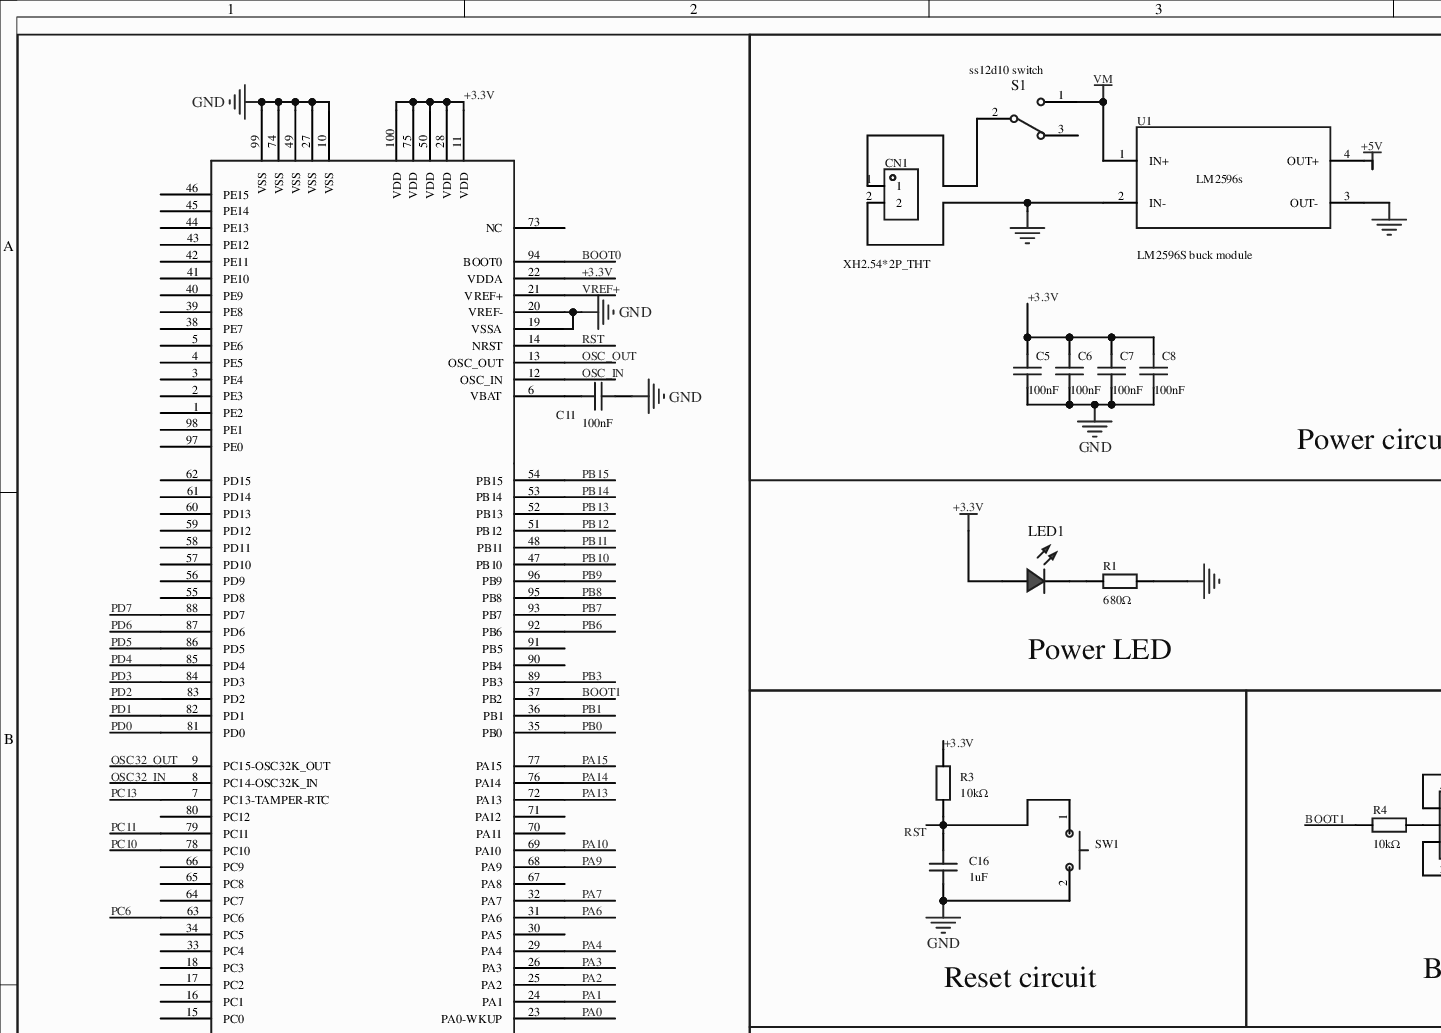
[diagram p0: MISC62445-3.schdoc, top left]
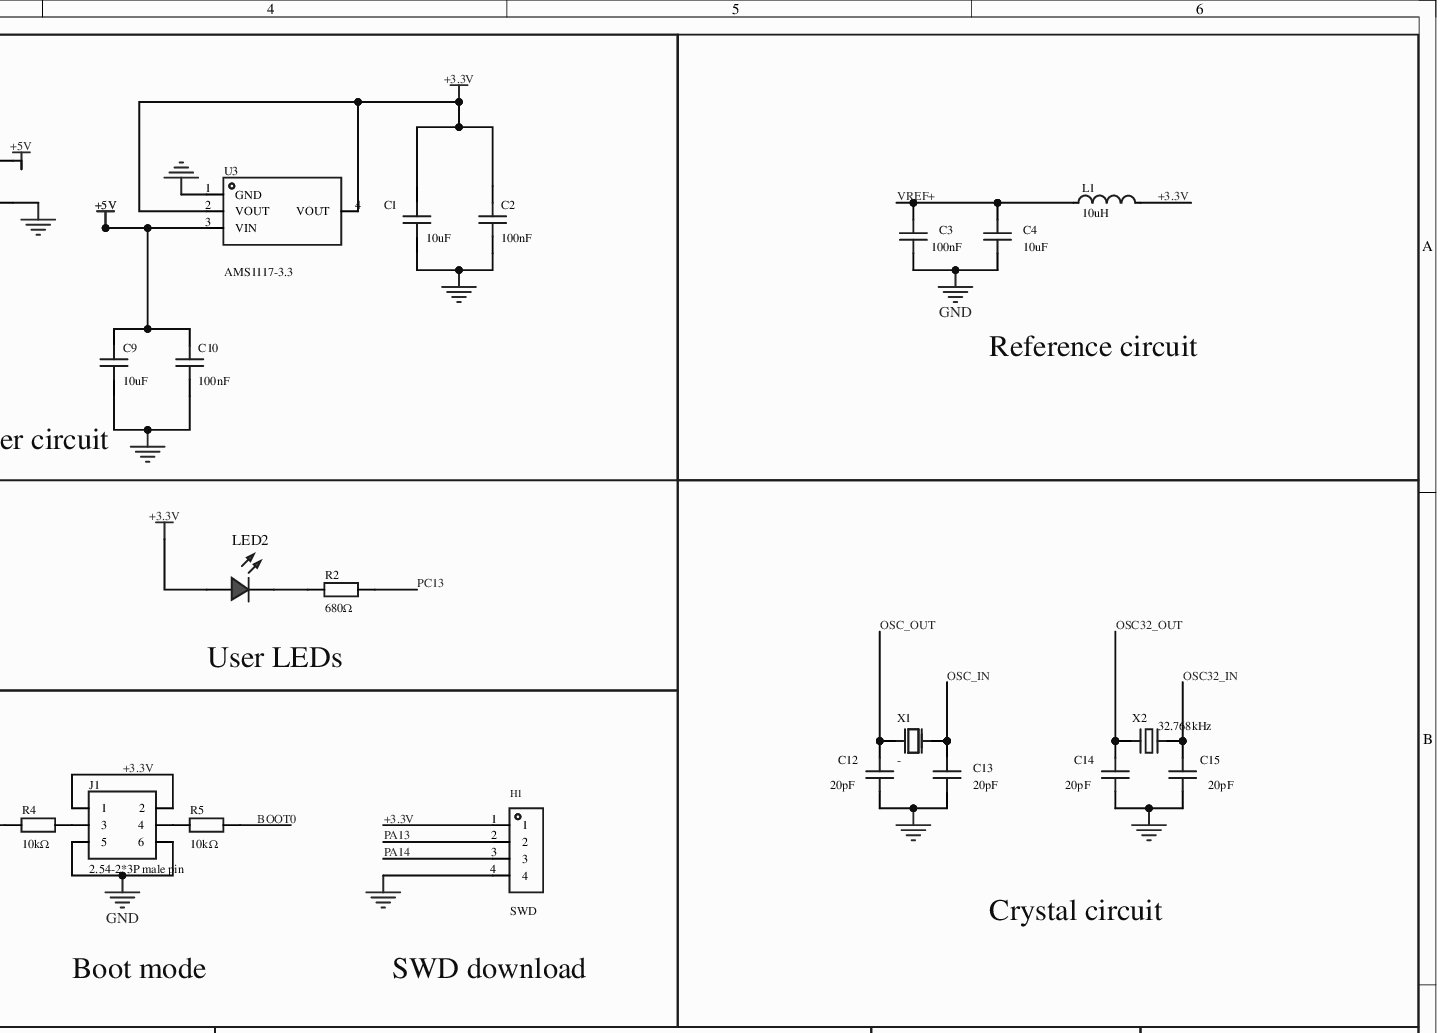
[diagram p1: MISC62445-3.schdoc, top right]
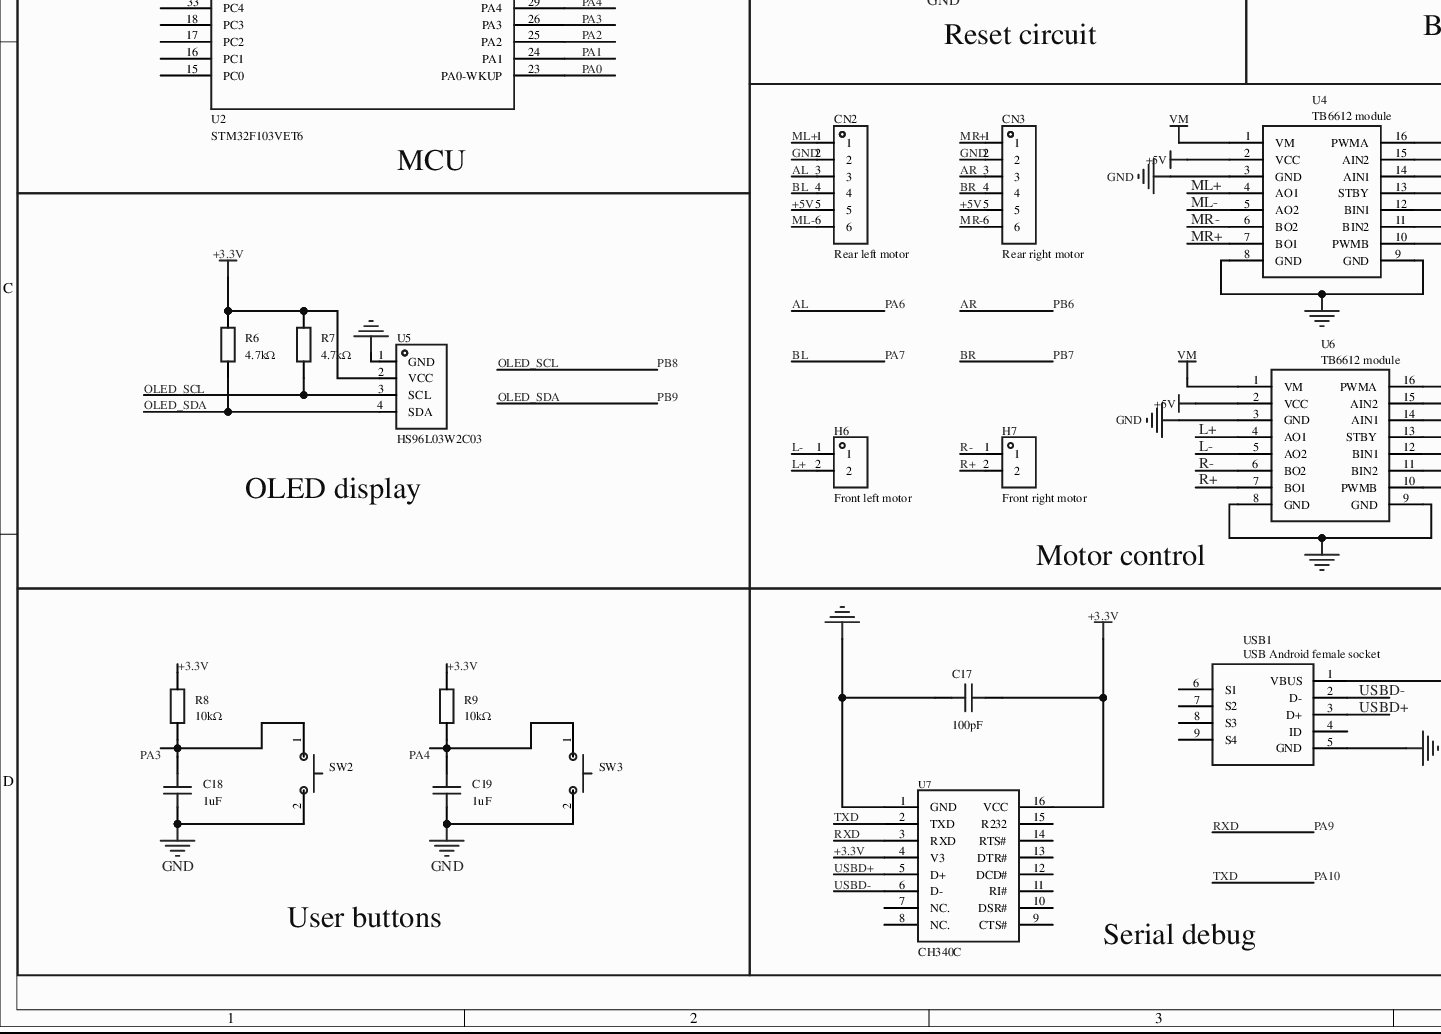
[diagram p2: MISC62445-3.schdoc, bottom left]
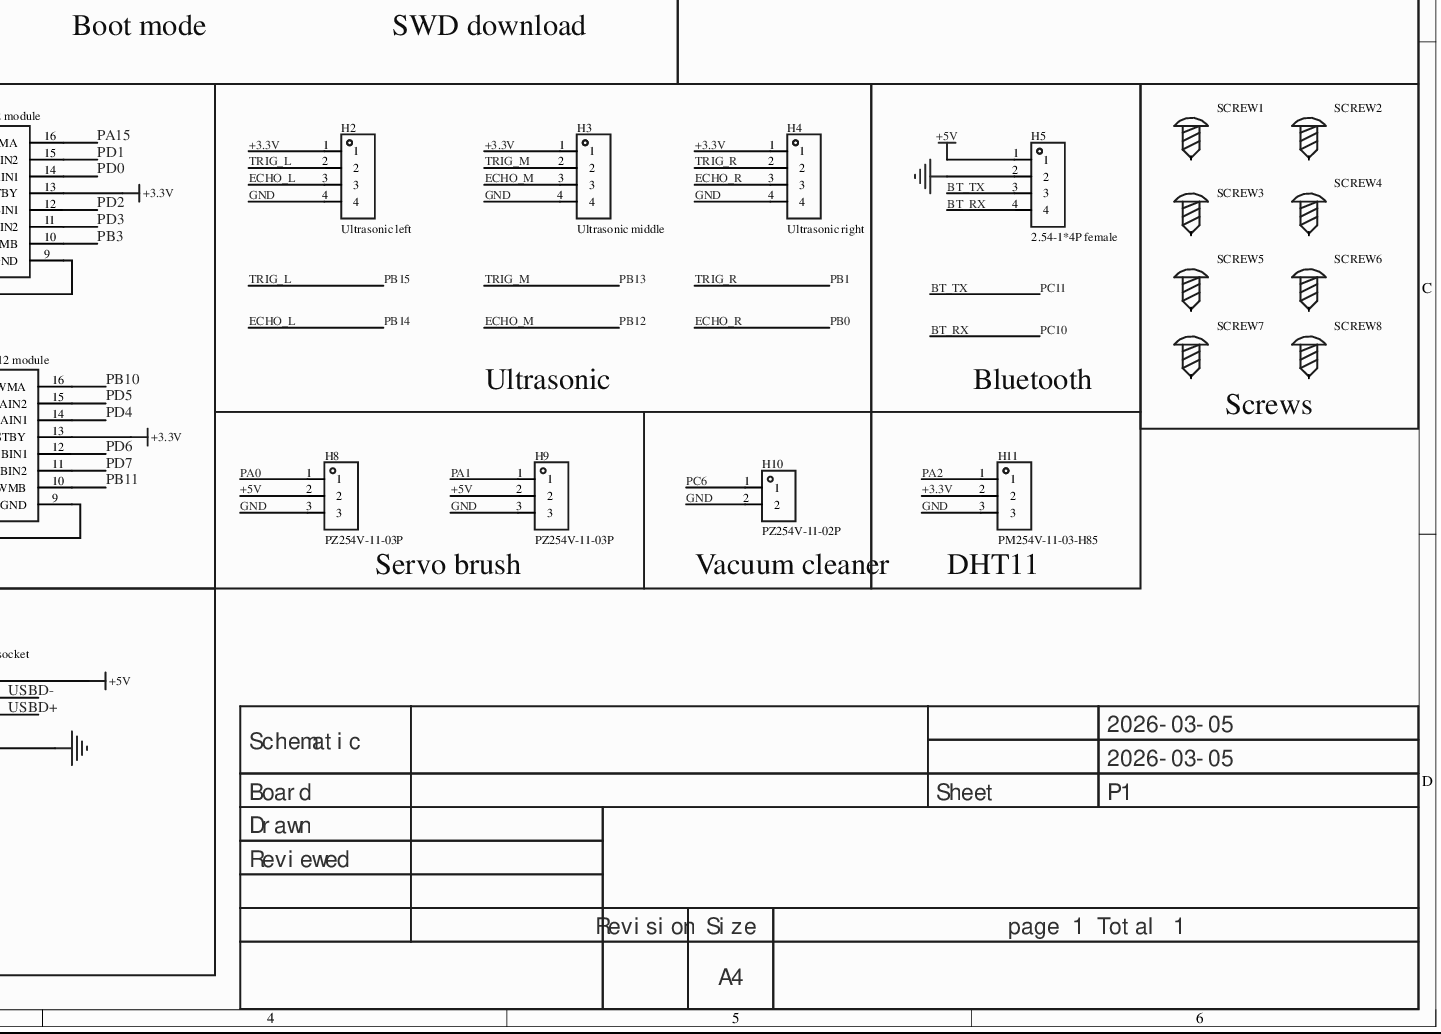
[diagram p3: MISC62445-3.schdoc, bottom right]
# Altium project MISC62445-2.PrjPcb
1 sheet, 68 parts. Net scope: global (net labels, ports and power ports of the same name join across sheets).
Board file: MISC62445.pcbdoc

## Sheet MISC62445-3.schdoc
size 420 x 297 mm; Version: V1.0; @Project Name: MISC62445; @Page Count: 1; @Update Date: 2026-03-05; @Create Date: 2026-03-05; @Schematic Name: MISC62445; @Page No: 1; @Create Time: 17:18:42; @Update Time: 10:03:47; @Board Name: MISC62445

### Parts
C1  10uF  [C0805]
C2  100nF  [C0805]
C3  100nF  [C0603]
C4  10uF  [C0603]
C5  100nF  [C0603]
C6  100nF  [C0603]
C7  100nF  [C0603]
C8  100nF  [C0603]
C9  10uF  [C0805]
C10  100nF  [C0805]
C11  100nF  [C0603]
C12  20pF  [C0805]
C13  20pF  [C0805]
C14  20pF  [C0805]
C15  20pF  [C0805]
C16  1uF  [C0603]
C17  100pF  [C0805]
C18  1uF  [C0603]
C19  1uF  [C0603]
CN1  XH2.54*2P_THT  [CONN-TH_2P-P2.50-XH2.54-2P]
CN2  Rear left motor  [CONN-TH_XH2.54-6P]
CN3  Rear right motor  [CONN-TH_XH2.54-6P]
H1  SWD  [HDR-TH_4P-P2.54-V-M]
H2  Ultrasonic left  [HDR-TH_4P-P2.54-V-M]
H3  Ultrasonic middle  [HDR-TH_4P-P2.54-V-M]
H4  Ultrasonic right  [HDR-TH_4P-P2.54-V-M]
H5  2.54-1*4P female  [HDR-TH_4P-P2.54-V-F]
H6  Front left motor  [HDR-TH_2P-P2.54-V-M]
H7  Front right motor  [HDR-TH_2P-P2.54-V-M]
H8  PZ254V-11-03P  [HDR-TH_3P-P2.54-V-M]
H9  PZ254V-11-03P  [HDR-TH_3P-P2.54-V-M]
H10  PZ254V-11-02P  [HDR-TH_2P-P2.54-V-M]
H11  PM254V-11-03-H85  [HDR-TH_3P-P2.54-V-F]
J1  2.54-2*3P male pin  [HDR-TH_6P-P2.54-V-M-R2-C3-S2.54-1]
L1  10uH  [L0603]
LED1  NCD0805R1  [LED0805-RD_RED]  (value not drawn)
LED2  NCD0805R1  [LED0805-RD_RED]  (value not drawn)
R1  680Ω  [R0805]
R2  680Ω  [R0805]
R3  10kΩ  [R0603]
R4  10kΩ  [R0603]
R5  10kΩ  [R0603]
R6  4.7kΩ  [R0805]
R7  4.7kΩ  [R0805]
R8  10kΩ  [R0603]
R9  10kΩ  [R0603]
S1  ss12d10 switch  [SS12D10]
SCREW1  (no value)  [M3螺丝]
SCREW2  (no value)  [M3螺丝]
SCREW3  (no value)  [M3螺丝]
SCREW4  (no value)  [M3螺丝]
SCREW5  (no value)  [M2螺丝]
SCREW6  (no value)  [M2螺丝]
SCREW7  (no value)  [M2螺丝]
SCREW8  (no value)  [M2螺丝]
SW1  1TS002C-2300-4300-CT  [SW-SMD_L6.0-W3.5-LS8.0-EH]  (value not drawn)
SW2  1TS002C-2300-4300-CT  [SW-SMD_L6.0-W3.5-LS8.0-EH]  (value not drawn)
SW3  1TS002C-2300-4300-CT  [SW-SMD_L6.0-W3.5-LS8.0-EH]  (value not drawn)
U1  LM2596S buck module  [LM2596S]
U2  STM32F103VET6  [LQFP-100_L14.0-W14.0-P0.50-LS16.0-BL]
U3  AMS1117-3.3  [SOT-223-3_L6.5-W3.4-P2.30-LS7.0-BR]
U4  TB6612 module  [TB6612-2X8]
U5  HS96L03W2C03  [OLED-TH_L27.8-W27.2-P2.54_C9900033791]
U6  TB6612 module  [TB6612-2X8]
U7  CH340C  [SOP-16_L10.0-W3.9-P1.27-LS6.0-BL]
USB1  USB Android female socket  [MICRO-USB-SMD_MICRO-USB-A8]
X1  -  [HC-49US_L11.5-W4.5-P4.88]
X2  32.768kHz  [OSC-SMD_L3.2-W1.5]

### Blocks framed on the sheet
MCU: C11 U2
Power circuit: C1 C2 C5-C10 CN1 S1 U1 U3
Reference circuit: C3 C4 L1
Crystal circuit: C12-C15 X1 X2
Reset circuit: C16 R3 SW1
Motor control: CN2 CN3 H6 H7 U4 U6
Ultrasonic: H2-H4
Bluetooth: H5
Screws: SCREW1-SCREW8
Vacuum cleaner: H10
User buttons: C18 C19 R8 R9 SW2 SW3

### Nets
+3.3V: C1.2 C2.2 C5.1 C6.1 C7.1 C8.1 C17.2 H1.1 H2.1 H3.1 H4.1 H11.2 J1.1 J1.2 L1.2 LED1.2(A) LED2.2(A) R3.2 R6.1 R7.1 R8.2 R9.2 U2.11(VDD) U2.22(VDDA) U2.28(VDD) U2.50(VDD) U2.75(VDD) U2.100(VDD) U3.2(VOUT) U3.4(VOUT) U4.13(STBY) U5.2(VCC) U6.13(STBY) U7.4(V3) U7.16(VCC)
+5V: C9.2 C10.2 CN2.5 CN3.5 H5.1 H8.2 H9.2 U1.4(OUT+) U3.3(VIN) U4.2(VCC) U6.2(VCC) USB1.1(VBUS)
GND: C1.1 C2.1 C3.1 C4.1 C5.2 C6.2 C7.2 C8.2 C9.1 C10.1 C11.2 C12.1 C13.1 C14.1 C15.1 C16.1 C17.1 C18.1 C19.1 CN1.2 CN2.2 CN3.2 H1.4 H2.4 H3.4 H4.4 H5.2 H8.3 H9.3 H10.2 H11.3 J1.5 J1.6 R1.2 SW1.2(B) SW2.2(B) SW3.2(B) U1.2(IN-) U1.3(OUT-) U2.10(VSS) U2.19(VSSA) U2.20(VREF-) U2.27(VSS) U2.49(VSS) U2.74(VSS) U2.99(VSS) U3.1(GND) U4.3(GND) U4.8(GND) U4.9(GND) U5.1(GND) U6.3(GND) U6.8(GND) U6.9(GND) U7.1(GND) USB1.5(GND)
VM: S1.1 U1.1(IN+) U4.1(VM) U6.1(VM)
AL: CN2.3 U2.31(PA6)  [also labelled PA6]
AR: CN3.3 U2.92(PB6)  [also labelled PB6]
BL: CN2.4 U2.32(PA7)  [also labelled PA7]
BOOT0: R5.2 U2.94(BOOT0)
BOOT1: R4.1 U2.37(PB2)
BR: CN3.4 U2.93(PB7)  [also labelled PB7]
BT_RX: H5.4 U2.78(PC10)  [also labelled PC10]
BT_TX: H5.3 U2.79(PC11)  [also labelled PC11]
ECHO_L: H2.3 U2.53(PB14)  [also labelled PB14]
ECHO_M: H3.3 U2.51(PB12)  [also labelled PB12]
ECHO_R: H4.3 U2.35(PB0)  [also labelled PB0]
L+: H6.2 U6.4(AO1)
L-: H6.1 U6.5(AO2)
ML+: CN2.1 U4.4(AO1)
ML-: CN2.6 U4.5(AO2)
MR+: CN3.1 U4.7(BO1)
MR-: CN3.6 U4.6(BO2)
OLED_SCL: R7.2 U2.95(PB8) U5.3(SCL)  [also labelled PB8]
OLED_SDA: R6.2 U2.96(PB9) U5.4(SDA)  [also labelled PB9]
OSC32_IN: C15.2 U2.8(PC14-OSC32K_IN) X2.2
OSC32_OUT: C14.2 U2.9(PC15-OSC32K_OUT) X2.1
OSC_IN: C13.2 U2.12(OSC_IN) X1.2(OSC2)
OSC_OUT: C12.2 U2.13(OSC_OUT) X1.1(OSC1)
PA0: H8.1 U2.23(PA0-WKUP)
PA1: H9.1 U2.24(PA1)
PA2: H11.1 U2.25(PA2)
PA3: C18.2 R8.1 SW2.1(A) U2.26(PA3)
PA4: C19.2 R9.1 SW3.1(A) U2.29(PA4)
PA9: U2.68(PA9) U7.3(RXD)  [also labelled RXD]
PA10: U2.69(PA10) U7.2(TXD)  [also labelled TXD]
PA13: H1.2 U2.72(PA13)
PA14: H1.3 U2.76(PA14)
PA15: U2.77(PA15) U4.16(PWMA)
PB1: H4.2 U2.36(PB1)  [also labelled TRIG_R]
PB3: U2.89(PB3) U4.10(PWMB)
PB10: U2.47(PB10) U6.16(PWMA)
PB11: U2.48(PB11) U6.10(PWMB)
PB13: H3.2 U2.52(PB13)  [also labelled TRIG_M]
PB15: H2.2 U2.54(PB15)  [also labelled TRIG_L]
PC6: H10.1 U2.63(PC6)
PC13: R2.2 U2.7(PC13-TAMPER-RTC)
PD0: U2.81(PD0) U4.14(AIN1)
PD1: U2.82(PD1) U4.15(AIN2)
PD2: U2.83(PD2) U4.12(BIN1)
PD3: U2.84(PD3) U4.11(BIN2)
PD4: U2.85(PD4) U6.14(AIN1)
PD5: U2.86(PD5) U6.15(AIN2)
PD6: U2.87(PD6) U6.12(BIN1)
PD7: U2.88(PD7) U6.11(BIN2)
R+: H7.2 U6.7(BO1)
R-: H7.1 U6.6(BO2)
RST: C16.2 R3.1 SW1.1(A) U2.14(NRST)
USBD+: U7.5(D+) USB1.3(D+)
USBD-: U7.6(D-) USB1.2(D-)
VREF+: C3.2 C4.2 L1.1 U2.21(VREF+)
NetC11_1: C11.1 U2.6(VBAT)
NetCN1_1: CN1.1 S1.2
NetJ1_3: J1.3 R4.2
NetJ1_4: J1.4 R5.1
NetLED1_1: LED1.1(C) R1.1
NetLED2_1: LED2.1(C) R2.1

Not connected (* = marked no-connect by the designer): S1 3*; SCREW1 1*; SCREW2 1*; SCREW3 1*; SCREW4 1*; SCREW5 1*; SCREW6 1*; SCREW7 1*; SCREW8 1*; U2 1(PE2)* 2(PE3)* 3(PE4)* 4(PE5)* 5(PE6)* 15(PC0)* 16(PC1)* 17(PC2)* 18(PC3)* 30(PA5)* 33(PC4)* 34(PC5)* 38(PE7)* 39(PE8)* 40(PE9)* 41(PE10)* 42(PE11)* 43(PE12)* 44(PE13)* 45(PE14)* 46(PE15)* 55(PD8)* 56(PD9)* 57(PD10)* 58(PD11)* 59(PD12)* 60(PD13)* 61(PD14)* 62(PD15)* 64(PC7)* 65(PC8)* 66(PC9)* 67(PA8)* 70(PA11)* 71(PA12)* 73(NC)* 80(PC12)* 90(PB4)* 91(PB5)* 97(PE0)* 98(PE1)*; U7 7(NC.)* 8(NC.)* 9(CTS#)* 10(DSR#)* 11(RI#)* 12(DCD#)* 13(DTR#)* 14(RTS#)* 15(R232)*; USB1 4(ID)* 6(S1)* 7(S2)* 8(S3)* 9(S4)*

### Notes on the sheet
- Power LED
- User LEDs
- Boot mode
- SWD download
- (near U5) OLED display
- (near H9) Servo brush
- (near H11) DHT11
- Serial debug
- 2026-03-05
- Schematic
- Board
- Sheet
- P1
- Drawn
- Reviewed
- Revision
- Size
- A4
- page 1 Total 1

### Library data of the parts
C1 C9 = GRM21BR61H106KE43L: Capacitance:10uF;Tolerance:±10%;Rated voltage:50V;Dielectric (temp. coeff.):X5R;; Manufacturer: muRata(村田); AddInBom: yes; ModelId: 1ba041120af144c991958decab20d241; ModelName: C0805_L2.0-W1.3-H1.3; ModelTransform: 78.74,51.181,0,0,0,0,0,0.0005,0; Tolerance: ±10%; Voltage Rated: 50V; Temperature Coefficient: X5R; Symbol: CapAcitance; Device: GRM21BR61H106KE43L; LCSC Part Name: 10uF ±10% 50V; SupplierPart: C440198; ManufacturerPart: GRM21BR61H106KE43L; Supplier Footprint: 0805; JLCPCB Part Class: Basic Part; Datasheet: https://example.com/upload/public/pdf/source/20230811/95AAE0C9AF55EDC31B7A4D8B733F534E.pdf; Supplier: LCSC; ConvertToPcb: yes; FootprintName: C0805; Value: 10uF
C2 C10 = CL21B104KBCNNNC: Capacitance:100nF;Tolerance:±10%;Rated voltage:50V;Dielectric (temp. coeff.):X7R;; Manufacturer: SAMSUNG(三星); AddInBom: yes; ModelId: 1ba041120af144c991958decab20d241; ModelName: C0805_L2.0-W1.3-H1.3; ModelTransform: 78.74,51.181,0,0,0,0,0,0.0005,0; Tolerance: ±10%; Voltage Rated: 50V; Temperature Coefficient: X7R; Symbol: CapAcitance; Device: CL21B104KBCNNNC; LCSC Part Name: 100nF ±10% 50V; SupplierPart: C1711; ManufacturerPart: CL21B104KBCNNNC; Supplier Footprint: 0805; JLCPCB Part Class: Extended Part; Datasheet: https://example.com/upload/public/pdf/source/20160218/1457707763339.pdf; Supplier: LCSC; ConvertToPcb: yes; FootprintName: C0805; Value: 100nF
C3 C5-C8 C11 = CC0603KRX7R9BB104: Capacitance:100nF;Tolerance:±10%;Rated voltage:50V;Dielectric (temp. coeff.):X7R;; Manufacturer: YAGEO(国巨); Check: true; AddInBom: yes; ModelId: ac125912035d415993ca9572d50418b1; ModelName: C0603_L1.6-W0.8-H0.8; ModelTransform: 62.992,31.496,0,0,0,0,0,0,0; Tolerance: ±10%; Voltage Rated: 50V; Temperature Coefficient: X7R; Symbol: CapAcitance; Device: CC0603KRX7R9BB104; Supplier Part: C14663; LCSC Part Name: 100nF ±10% 50V; ManufacturerPart: CC0603KRX7R9BB104; Supplier Footprint: 0603; JLCPCB Part Class: Basic Part; Datasheet: https://example.com/upload/public/pdf/source/20180910/C282072_33301C7F631E79921B82A8DAC6BCC5B3.pdf; Supplier: LCSC; ConvertToPcb: yes; FootprintName: C0603; Value: 100nF
C4 = CL10A106KP8NNNC: Capacitance:10uF;Tolerance:±10%;Rated voltage:10V;Dielectric:X5R;; Manufacturer: SAMSUNG(三星); Check: true; AddInBom: yes; ModelId: ac125912035d415993ca9572d50418b1; ModelName: C0603_L1.6-W0.8-H0.8; ModelTransform: 62.992,31.496,0,0,0,0,0,0,0; Tolerance: ±10%; Voltage Rated: 10V; Temperature Coefficient: X5R; Symbol: CapAcitance; Device: CL10A106KP8NNNC; Supplier Part: C19702; LCSC Part Name: 10uF ±10% 10V; ManufacturerPart: CL10A106KP8NNNC; Supplier Footprint: 0603; JLCPCB Part Class: Basic Part; Datasheet: https://example.com/upload/public/pdf/source/20160103/1457707703378.pdf; Supplier: LCSC; ConvertToPcb: yes; FootprintName: C0603; Value: 10uF
C12-C15 = CL21C200JBANNNC: Capacitance:20pF;Tolerance:±5%;Rated voltage:50V;Dielectric:C0G;; Manufacturer: SAMSUNG(三星); AddInBom: yes; ModelId: 1ba041120af144c991958decab20d241; ModelName: C0805_L2.0-W1.3-H1.3; ModelTransform: 78.74,51.181,0,0,0,0,0,0.0005,0; Tolerance: ±5%; Voltage Rated: 50V; Temperature Coefficient: C0G; Symbol: CapAcitance; Device: CL21C200JBANNNC; LCSC Part Name: 20pF ±5% 50V; SupplierPart: C1798; ManufacturerPart: CL21C200JBANNNC; Supplier Footprint: 0805; JLCPCB Part Class: Basic Part; Datasheet: https://example.com/upload/public/pdf/source/20160218/1457707763339.pdf; Supplier: LCSC; ConvertToPcb: yes; FootprintName: C0805; Value: 20pF
C16 C18 C19 = CL10A105KB8NNNC: Capacitance:1uF;Tolerance:±10%;Rated voltage:50V;Dielectric:X5R;; Manufacturer: SAMSUNG(三星); Check: true; AddInBom: yes; ModelId: ac125912035d415993ca9572d50418b1; ModelName: C0603_L1.6-W0.8-H0.8; ModelTransform: 62.992,31.496,0,0,0,0,0,0,0; Tolerance: ±10%; Voltage Rated: 50V; Temperature Coefficient: X5R; Symbol: CapAcitance; Device: CL10A105KB8NNNC; Supplier Part: C15849; LCSC Part Name: 1uF ±10% 50V; ManufacturerPart: CL10A105KB8NNNC; Supplier Footprint: 0603; JLCPCB Part Class: Basic Part; Datasheet: https://example.com/upload/public/pdf/source/20160103/1457707679084.pdf; Supplier: LCSC; ConvertToPcb: yes; FootprintName: C0603; Value: 1uF
C17 = CL21C101JBANNNC: Capacitance:100pF;Tolerance:±5%;Rated voltage:50V;Dielectric:C0G;; Manufacturer: SAMSUNG(三星); AddInBom: yes; ModelId: 1ba041120af144c991958decab20d241; ModelName: C0805_L2.0-W1.3-H1.3; ModelTransform: 78.74,51.181,0,0,0,0,0,0.0005,0; Tolerance: ±5%; Voltage Rated: 50V; Temperature Coefficient: C0G; Symbol: CapAcitance; Device: CL21C101JBANNNC; LCSC Part Name: 100pF ±5% 50V; SupplierPart: C1790; ManufacturerPart: CL21C101JBANNNC; Supplier Footprint: 0805; JLCPCB Part Class: Basic Part; Datasheet: https://example.com/upload/public/pdf/source/20160218/1457707763339.pdf; Supplier: LCSC; ConvertToPcb: yes; FootprintName: C0805; Value: 100pF
CN1 = XH2.54*2P_直插: Manufacturer: null; Convert to PCB: yes; ModelId: 325c595e30db4df8abe76612dd40b0fa; Origin Footprint: CONN-TH_2P-P2.50-XH2.54-2P; Device: XH2.54*2P_THT; Symbol: XH2.54*2P_THT; Supplier: LCSC; Supplier Part: C9900008615; Manufacturer Part: XH2.54*2P_直插; JLCPCB Part Class: Extended Part; Add into BOM: yes; FootprintName: CONN-TH_2P-P2.50-XH2.54-2P; link: https://example.com/pdf/applyPasteComponent/2021-09-13/837084A/aaafcbedaa1341f78bdd46f8ab13ab21/XH2_54datasheet.pdf; 3DModel: CONN-TH_2P-P2.50-XH2.54-2P; ModelName: CONN-TH_2P-P2.50-XH2.54-2P
CN2 = XH2.54*6P_直插: Manufacturer Part: 后左电机; Symbol: XH2.54*6P_THT; AddInBom: yes; ModelId: a7224aacb0dc4305a7392217f7fd8fe2; ModelTransform: 688.975,224.409,0,0,0,0,-0.001,-17.719,-118.11; Device: XH2.54*6P_THT; LCSC Part Name: XH2.54*6P_直插; SupplierPart: C9900008614; Supplier Footprint: XH2.54_6P; JLCPCB Part Class: Extended library; Supplier: LCSC; ConvertToPcb: yes; FootprintName: CONN-TH_XH2.54-6P; ModelName: CONN-TH_XH2.54-6P
CN3 = XH2.54*6P_直插: Manufacturer Part: 后右电机; Symbol: XH2.54*6P_THT; AddInBom: yes; ModelId: a7224aacb0dc4305a7392217f7fd8fe2; ModelTransform: 688.975,224.409,0,0,0,0,-0.001,-17.719,-118.11; Device: XH2.54*6P_THT; LCSC Part Name: XH2.54*6P_直插; SupplierPart: C9900008614; Supplier Footprint: XH2.54_6P; JLCPCB Part Class: Extended library; Supplier: LCSC; ConvertToPcb: yes; FootprintName: CONN-TH_XH2.54-6P; ModelName: CONN-TH_XH2.54-6P
H1 = KH-2.54PH180-1X4P-L11.5: 排数:单排;总PIN位数:4P;间距:2.54mm;插针结构:1x4P;行距:-;安装类型:直插;圆针/方针:方针;额定电流:3A;额定电压:-;配合针长度:6mm;塑高:2.5mm;端接针长度:3mm;触头材质:-;工作温度范围:-40℃~+105℃;颜色:黑色;; Manufacturer: kinghelm(金航标); AddInBom: yes; ModelId: 112f4d05e8d64e99ab9a333894bea4f9; ModelName: HDR-TH_4P-P2.54-M-LI-1X4P; ModelTransform: 399.999,104.7242,0,0,0,0,0,0,-118.11; Pitch: 2.54mm; Pin Structure: 1x4P; Circluar Pins/Square Pins: Square pin; Current Rating (Max): 3A; Symbol: KH-2.54PH180-1X4P-L11.5; Manufacturer Part: SWD; Device: KH-2.54PH180-1X4P-L11.5; Supplier: LCSC; Supplier Part: C2905435; JLCPCB Part Class: Extended Part; LCSC Part Name: 2.54mm 1x4P 直插 方针; Supplier Footprint: 插件,P=2.54mm; Datasheet: https://example.com/upload/public/pdf/source/20211019/06FD9EA041E66F176E900F61FE678D35.pdf; ConvertToPcb: yes; FootprintName: HDR-TH_4P-P2.54-V-M; Number of Rows: Single row; Number of Pins: 4P; Row Spacing: -; Mounting Type: Through-hole; Voltage Rating (Max): -; Length of Mating Pin: 6mm; Insulation Height: 2.5mm; Length of End Connection Pin: 3mm; Contact Material: -; Operating Temperature Range: -40℃~+105℃; Color: Black
H2 = PZ254V-11-04P: 插针结构:1x4P;间距:2.54mm;行距:-;圆针/方针:方针;安装类型:直插;排数:单排;总PIN位数:4P;额定电流:3A;额定电压:250V;配合针长度:6mm;塑高:2.5mm;端接针长度:3mm;触头材质:-;工作温度范围:-40℃~+105℃;颜色:黑色;; Manufacturer Part: 超声波左; Manufacturer: XFCN(兴飞); Symbol: PZ254V-11-04P_C2691448; AddInBom: yes; ModelId: 112f4d05e8d64e99ab9a333894bea4f9; ModelName: HDR-TH_4P-P2.54-M-LI-1X4P; ModelTransform: 399.999,104.7242,0,0,0,0,0,0,-118.11; Pin Structure: 1x4P; Pitch: 2.54mm; Circluar Pins/Square Pins: Square pin; Current Rating (Max): 3A; Voltage Rating (Max): 250V; Device: PZ254V-11-04P; LCSC Part Name: 间距:2.54mm 1x4P 直插 方针; SupplierPart: C2691448; Supplier Footprint: 插件,P=2.54mm; JLCPCB Part Class: Extended library; Datasheet: https://example.com/upload/public/pdf/source/20200309/C492403_F9F19131791D08044AD4F84F8E751A34.pdf; Supplier: LCSC; ConvertToPcb: yes; FootprintName: HDR-TH_4P-P2.54-V-M; Row Spacing: -; Mounting Type: Through-hole; Number of Rows: Single row; Number of Pins: 4P; Length of Mating Pin: 6mm; Insulation Height: 2.5mm; Length of End Connection Pin: 3mm; Contact Material: -; Operating Temperature Range: -40℃~+105℃; Color: Black
H3 = PZ254V-11-04P: 插针结构:1x4P;间距:2.54mm;行距:-;圆针/方针:方针;安装类型:直插;排数:单排;总PIN位数:4P;额定电流:3A;额定电压:250V;配合针长度:6mm;塑高:2.5mm;端接针长度:3mm;触头材质:-;工作温度范围:-40℃~+105℃;颜色:黑色;; Manufacturer Part: 超声波中; Manufacturer: XFCN(兴飞); Symbol: PZ254V-11-04P_C2691448; AddInBom: yes; ModelId: 112f4d05e8d64e99ab9a333894bea4f9; ModelName: HDR-TH_4P-P2.54-M-LI-1X4P; ModelTransform: 399.999,104.7242,0,0,0,0,0,0,-118.11; Pin Structure: 1x4P; Pitch: 2.54mm; Circluar Pins/Square Pins: Square pin; Current Rating (Max): 3A; Voltage Rating (Max): 250V; Device: PZ254V-11-04P; LCSC Part Name: 间距:2.54mm 1x4P 直插 方针; SupplierPart: C2691448; Supplier Footprint: 插件,P=2.54mm; JLCPCB Part Class: Extended library; Datasheet: https://example.com/upload/public/pdf/source/20200309/C492403_F9F19131791D08044AD4F84F8E751A34.pdf; Supplier: LCSC; ConvertToPcb: yes; FootprintName: HDR-TH_4P-P2.54-V-M; Row Spacing: -; Mounting Type: Through-hole; Number of Rows: Single row; Number of Pins: 4P; Length of Mating Pin: 6mm; Insulation Height: 2.5mm; Length of End Connection Pin: 3mm; Contact Material: -; Operating Temperature Range: -40℃~+105℃; Color: Black
H4 = PZ254V-11-04P: 插针结构:1x4P;间距:2.54mm;行距:-;圆针/方针:方针;安装类型:直插;排数:单排;总PIN位数:4P;额定电流:3A;额定电压:250V;配合针长度:6mm;塑高:2.5mm;端接针长度:3mm;触头材质:-;工作温度范围:-40℃~+105℃;颜色:黑色;; Manufacturer Part: 超声波右; Manufacturer: XFCN(兴飞); Symbol: PZ254V-11-04P_C2691448; AddInBom: yes; ModelId: 112f4d05e8d64e99ab9a333894bea4f9; ModelName: HDR-TH_4P-P2.54-M-LI-1X4P; ModelTransform: 399.999,104.7242,0,0,0,0,0,0,-118.11; Pin Structure: 1x4P; Pitch: 2.54mm; Circluar Pins/Square Pins: Square pin; Current Rating (Max): 3A; Voltage Rating (Max): 250V; Device: PZ254V-11-04P; LCSC Part Name: 间距:2.54mm 1x4P 直插 方针; SupplierPart: C2691448; Supplier Footprint: 插件,P=2.54mm; JLCPCB Part Class: Extended library; Datasheet: https://example.com/upload/public/pdf/source/20200309/C492403_F9F19131791D08044AD4F84F8E751A34.pdf; Supplier: LCSC; ConvertToPcb: yes; FootprintName: HDR-TH_4P-P2.54-V-M; Row Spacing: -; Mounting Type: Through-hole; Number of Rows: Single row; Number of Pins: 4P; Length of Mating Pin: 6mm; Insulation Height: 2.5mm; Length of End Connection Pin: 3mm; Contact Material: -; Operating Temperature Range: -40℃~+105℃; Color: Black
H5 = 2.54-1*4P母: 插孔结构:1x4P;间距:2.54mm;行距:-;圆孔/方孔:方孔;安装类型:直插;排数:单排;总孔位数:4P;额定电流:3A;额定电压:-;插孔方向:顶部;塑高:-;触头材质:青铜;触头镀层:-;工作温度范围:-40℃~+105℃;焊接温度(最大值):-;; Manufacturer: BOOMELE(博穆精密); AddInBom: yes; ModelId: d187812051054f85879fcaa51a310d8e; ModelTransform: 419.6842,98.464,0,0,0,0,0,0,-118.11; Holes Structure: 1x4P; Pitch: 2.54mm; Circular Hole / Square Hole: Square hole; Number of Holes: 4P; Current Rating (Max): 3A; Holes Direction: Top; Symbol: 2.54-1*4P female; Device: 2.54-1*4P female; LCSC Part Name: 间距:2.54mm 1x4P 直插; SupplierPart: C2718488; ManufacturerPart: 2.54-1*4P母; Supplier Footprint: 插件,P=2.54mm; JLCPCB Part Class: Extended library; Datasheet: https://example.com/upload/public/pdf/source/20210301/C2718488_F4427B881E42CAA8DDB0B1C12B3A522C.pdf; Supplier: LCSC; ConvertToPcb: yes; FootprintName: HDR-TH_4P-P2.54-V-F; ModelName: HDR-TH_4P-P2.54-V-F; Row Spacing: -; Mounting Type: Through-hole; Number of Rows: Single row; Voltage Rating (Max): -; Insulation Height: -; Contact Material: Bronze; Contact Plating: -; Operating Temperature Range: -40℃~+105℃; Soldering Temperature(Max): -
H6 = PZ254V-11-02P: 插针结构:1x2P;间距:2.54mm;行距:-;圆针/方针:方针;安装方式:直插;排数:单排;总PIN位数:2P;额定电流:-;额定电压:-;配合针长度:6mm;塑高:2.5mm;端接针长度:3mm;触头材质:黄铜;触头镀层:-;工作温度:-40℃~+105℃;颜色:黑色;; Manufacturer Part: 前左电机; Manufacturer: XFCN(兴飞); AddInBom: yes; ModelId: e35305ec3aa84b66b849f914b715e73f; ModelName: HDR2.54-M-LI-1X2P; ModelTransform: 200,100,0,0,0,0,0,0,-118.11; Pin Structure: 1x2P; Pitch: 2.54mm; Circluar Pins/Square Pins: Square pin; Symbol: PZ254V-11-02P; Device: PZ254V-11-02P; LCSC Part Name: 1x2P 间距:2.54mm 方针 直插; SupplierPart: C492401; Supplier Footprint: 插件,P=2.54mm; JLCPCB Part Class: Extended library; Datasheet: https://example.com/upload/public/pdf/source/20200309/C492401_A812433581A9B211A7FFA413ADDFF0E5.pdf; Supplier: LCSC; ConvertToPcb: yes; FootprintName: HDR-TH_2P-P2.54-V-M; Row Spacing: -; Mounting Type: Through-hole; Number of Rows: Single row; Number of Pins: 2P; Current Rating: -; Voltage Rating (Max): -; Length of Mating Pin: 6mm; Insulation Height: 2.5mm; Length of End Connection Pin: 3mm; Contact Material: Brass; Contact Plating: -; Operating Temperature: -40℃~+105℃; Color: Black
H7 = PZ254V-11-02P: 插针结构:1x2P;间距:2.54mm;行距:-;圆针/方针:方针;安装方式:直插;排数:单排;总PIN位数:2P;额定电流:-;额定电压:-;配合针长度:6mm;塑高:2.5mm;端接针长度:3mm;触头材质:黄铜;触头镀层:-;工作温度:-40℃~+105℃;颜色:黑色;; Manufacturer Part: 前右电机; Manufacturer: XFCN(兴飞); AddInBom: yes; ModelId: e35305ec3aa84b66b849f914b715e73f; ModelName: HDR2.54-M-LI-1X2P; ModelTransform: 200,100,0,0,0,0,0,0,-118.11; Pin Structure: 1x2P; Pitch: 2.54mm; Circluar Pins/Square Pins: Square pin; Symbol: PZ254V-11-02P; Device: PZ254V-11-02P; LCSC Part Name: 1x2P 间距:2.54mm 方针 直插; SupplierPart: C492401; Supplier Footprint: 插件,P=2.54mm; JLCPCB Part Class: Extended library; Datasheet: https://example.com/upload/public/pdf/source/20200309/C492401_A812433581A9B211A7FFA413ADDFF0E5.pdf; Supplier: LCSC; ConvertToPcb: yes; FootprintName: HDR-TH_2P-P2.54-V-M; Row Spacing: -; Mounting Type: Through-hole; Number of Rows: Single row; Number of Pins: 2P; Current Rating: -; Voltage Rating (Max): -; Length of Mating Pin: 6mm; Insulation Height: 2.5mm; Length of End Connection Pin: 3mm; Contact Material: Brass; Contact Plating: -; Operating Temperature: -40℃~+105℃; Color: Black
H8 H9 = PZ254V-11-03P: 插针结构:1x3P;间距:2.54mm;行距:-;圆针/方针:方针;安装方式:直插;排数:单排;总PIN位数:3P;额定电流:3A;额定电压:250V;配合针长度:6mm;塑高:2.5mm;端接针长度:3mm;工作温度:-40℃~+105℃;颜色:黑色;; Manufacturer: XFCN(兴飞); Symbol: PZ254V-11-03P_C2937625; AddInBom: yes; ModelId: bb473b6d38ff42a99216a4fcdbdcc4cb; ModelName: HDR-TH_3P-P2.54-M-LI-1X3P; ModelTransform: 299.9994,100,0,0,0,0,0,0,-118.11; Pin Structure: 1x3P; Pitch: 2.54mm; Circluar Pins/Square Pins: Square pin; Current Rating: 3A; Voltage Rating (Max): 250V; Device: PZ254V-11-03P; LCSC Part Name: 1x3P 间距:2.54mm 方针 直插; SupplierPart: C2937625; ManufacturerPart: PZ254V-11-03P; Supplier Footprint: 插件,P=2.54mm; JLCPCB Part Class: Extended library; Datasheet: https://example.com/upload/public/pdf/source/20200309/C492402_8335C3D49C4E4C618838D59BB1D024C1.pdf; Supplier: LCSC; ConvertToPcb: yes; FootprintName: HDR-TH_3P-P2.54-V-M; Row Spacing: -; Mounting Type: Through-hole; Number of Rows: Single row; Number of Pins: 3P; Length of Mating Pin: 6mm; Insulation Height: 2.5mm; Length of End Connection Pin: 3mm; Operating Temperature: -40℃~+105℃; Color: Black
H10 = PZ254V-11-02P: 插针结构:1x2P;间距:2.54mm;行距:-;圆针/方针:方针;安装方式:直插;排数:单排;总PIN位数:2P;额定电流:-;额定电压:-;配合针长度:6mm;塑高:2.5mm;端接针长度:3mm;触头材质:黄铜;触头镀层:-;工作温度:-40℃~+105℃;颜色:黑色;; Manufacturer: XFCN(兴飞); AddInBom: yes; ModelId: e35305ec3aa84b66b849f914b715e73f; ModelName: HDR2.54-M-LI-1X2P; ModelTransform: 200,100,0,0,0,0,0,0,-118.11; Pin Structure: 1x2P; Pitch: 2.54mm; Circluar Pins/Square Pins: Square pin; Symbol: PZ254V-11-02P; Device: PZ254V-11-02P; LCSC Part Name: 1x2P 间距:2.54mm 方针 直插; SupplierPart: C492401; ManufacturerPart: PZ254V-11-02P; Supplier Footprint: 插件,P=2.54mm; JLCPCB Part Class: Extended library; Datasheet: https://example.com/upload/public/pdf/source/20200309/C492401_A812433581A9B211A7FFA413ADDFF0E5.pdf; Supplier: LCSC; ConvertToPcb: yes; FootprintName: HDR-TH_2P-P2.54-V-M; Row Spacing: -; Mounting Type: Through-hole; Number of Rows: Single row; Number of Pins: 2P; Current Rating: -; Voltage Rating (Max): -; Length of Mating Pin: 6mm; Insulation Height: 2.5mm; Length of End Connection Pin: 3mm; Contact Material: Brass; Contact Plating: -; Operating Temperature: -40℃~+105℃; Color: Black
H11 = PM254V-11-03-H85: Socket structure:1x3P;Pitch:2.54mm;Row spacing:-;Mounting type:Through-hole;Rows:Single;Total hole count:3P;Plastic height:-;Contact material:Brass;Contact plating:-;; Manufacturer: XFCN(兴飞); AddInBom: yes; ModelId: f3b3cc5aae9641bf9e56fc160cef875b; ModelName: HDR2.54-F-LI-1X3P; ModelTransform: 299.9994,100,0,0,0,0,0,0,-118.11; Holes Structure: 1x3P; Pitch: 2.54mm; Number of Holes: 3P; Symbol: PM254V-11-03-H85; Device: PM254V-11-03-H85; LCSC Part Name: 间距:2.54mm 1x3P 直插; SupplierPart: C541850; ManufacturerPart: PM254V-11-03-H85; Supplier Footprint: 插件,P=2.54mm; JLCPCB Part Class: Extended library; Datasheet: https://example.com/upload/public/pdf/source/20200518/C541849_85853D71FC67C51915A806977A588FDA.pdf; Supplier: LCSC; ConvertToPcb: yes; FootprintName: HDR-TH_3P-P2.54-V-F; Row Spacing: -; Mounting Type: Through-hole; Number of Rows: Single row; Insulation Height: -; Contact Material: Brass; Contact Plating: -
J1 = 2.54-2*3P针: 排数:双排;总PIN位数:6;间距:2.54mm;插针结构:-;行距:-;安装类型:直插;圆针/方针:-;额定电流:-;额定电压:-;配合针长度:-;塑高:-;触头材质:-;触头镀层:-;颜色:黑色;; Manufacturer: BOOMELE(博穆精密); Check: true; Symbol: Header-Male-2.54_2x3; AddInBom: yes; ModelId: fd1b55b786fb415ca65c4187088147b7; ModelName: HDR2.54-M-LI-2x3P; ModelTransform: 299.9994,200,0,0,0,0,0,0,-118.11; Pitch: 2.54mm; Device: 2.54-2*3P male pin; LCSC Part Name: 2.54mm 直插; SupplierPart: C65114; ManufacturerPart: 2.54-2*3P针; Supplier Footprint: 插件,P=2.54mm; JLCPCB Part Class: Extended Part; Datasheet: https://example.com/upload/public/pdf/source/20221201/C605E3BE9C0F7226363017EFD1BDE852.pdf; Supplier: LCSC; ConvertToPcb: yes; FootprintName: HDR-TH_6P-P2.54-V-M-R2-C3-S2.54-1; Number of Rows: Dual row; Number of Pins: 6; Pin Structure: -; Row Spacing: -; Mounting Type: Through-hole; Circluar Pins/Square Pins: -; Current Rating (Max): -; Voltage Rating (Max): -; Length of Mating Pin: -; Insulation Height: -; Contact Material: -; Contact Plating: -; Color: Black
L1 = SDFL1608S100KTF: Inductance:10uH;Tolerance:±10%;Rated current:3mA;Saturation current (Isat):-;DC resistance (DCR):1.85Ω;; Manufacturer: Sunlord(顺络); Check: true; AddInBom: yes; ModelId: 2bc5ec593d464d6ba9807aec0b5673c2; ModelName: L0603_L1.6-W0.8-H0.5_BEAD; ModelTransform: 62.992,31.496,0,180,0,0,0.094,0.629,0; Tolerance: ±10%; Rated Current: 3mA; DC Resistance (DCR): 1.85Ω; Q @ Freq: 30@2MHz; Frequency - Self Resonant: 2MHz; Device: SDFL1608S100KTF; Symbol: SDFL1608S100KTF; LCSC Part Name: 10uH ±10% 1.85Ω; SupplierPart: C1035; ManufacturerPart: SDFL1608S100KTF; Supplier Footprint: 0603; JLCPCB Part Class: Basic Part; Datasheet: https://example.com/upload/public/pdf/source/20210816/855F4348312D259031B87CBCF31BE802.pdf; Supplier: LCSC; ConvertToPcb: yes; FootprintName: L0603; Value: 10uH; Saturation Current (Isat): -; Ratings: -
LED1 LED2 = NCD0805R1: Emitted color:Red;; Manufacturer: 国星光电; Symbol: LED_R; Convert to PCB: yes; 3D Model: 9e1095fac56a47ba900124c2261595bd; 3D Model Transform: 79.527,49.2125,0,0,0,0,0,0,0; Emitted Color: Red; Device: NCD0805R1; Add into BOM: yes; Supplier Footprint: 0805; Supplier Part: C84256; JLCPCB Part Class: Basic Part; LCSC Part Name: 红灯; ManufacturerPart: NCD0805R1; Datasheet: https://example.com/upload/public/pdf/source/20200820/C84256_F0A75A43B3EAD75808600A0514C76B99.pdf; Supplier: LCSC; FootprintName: LED0805-RD_RED; ModelName: LED0805-RD_RED
R1 R2 = 0805W8F6800T5E: Resistor type:Thick-film resistor;Resistance:680Ω;Tolerance:±1%;Power:125mW;Max working voltage:150V;Temp. coeff.:±100ppm/℃;; Manufacturer: UNI-ROYAL(厚声); AddInBom: yes; ModelId: 37a81e68749a4138bd2dfa6897b24b85; ModelName: R0805_L2.0-W1.3-H0.6; ModelTransform: 78.74,51.181,0,0,0,0,0,-0.0005,0; Tolerance: ±1%; Power(Watts): 125mW; Overload Voltage (Max): 150V; Symbol: Resistor; Device: 0805W8F6800T5E; LCSC Part Name: 680Ω ±1% 125mW 厚膜电阻; SupplierPart: C17798; ManufacturerPart: 0805W8F6800T5E; Supplier Footprint: 0805; JLCPCB Part Class: Basic Part; Datasheet: https://example.com/upload/public/pdf/source/20200306/C422600_1E6D84923E4A46A82E41ADD87F860B5C.pdf; Supplier: LCSC; ConvertToPcb: yes; FootprintName: R0805; Type: Thick-film resistor; Value: 680Ω; Temperature Coefficient: ±100ppm/℃; Operating Temperature Range: -55℃~+155℃
R3-R5 R8 R9 = 0603WAF1002T5E: Resistor type:Thick-film resistor;Resistance:10kΩ;Tolerance:±1%;Power:100mW;; Manufacturer: UNI-ROYAL(厚声); Check: true; AddInBom: yes; ModelId: fc143cca1e79419f9cd78b61e9279f08; ModelTransform: 31.8897,63.7794,0,90,0,0,0,0,0; Tolerance: ±1%; Power(Watts): 100mW; Temperature Coefficient: ±100ppm/℃; Overload Voltage (Max): 75V; Symbol: Resistor; Device: 0603WAF1002T5E; LCSC Part Name: 10kΩ ±1% 100mW; SupplierPart: C25804; ManufacturerPart: 0603WAF1002T5E; Supplier Footprint: 0603; JLCPCB Part Class: Basic Part; Datasheet: https://example.com/upload/public/pdf/source/20200306/C422600_1E6D84923E4A46A82E41ADD87F860B5C.pdf; Supplier: LCSC; ConvertToPcb: yes; FootprintName: R0603; ModelName: R0603; Type: Thick-film resistor; Value: 10kΩ; Operating Temperature Range: -55℃~+155℃
R6 R7 = 0805W8F4701T5E: Resistor type:Thick-film resistor;Resistance:4.7kΩ;Tolerance:±1%;Power:125mW;Max working voltage:150V;Temp. coeff.:±100ppm/℃;; Manufacturer: UNI-ROYAL(厚声); AddInBom: yes; ModelId: 37a81e68749a4138bd2dfa6897b24b85; ModelName: R0805_L2.0-W1.3-H0.6; ModelTransform: 78.74,51.181,0,0,0,0,0,-0.0005,0; Tolerance: ±1%; Power(Watts): 125mW; Overload Voltage (Max): 150V; Symbol: 0805W8F4701T5E; Device: 0805W8F4701T5E; LCSC Part Name: 4.7kΩ ±1% 125mW 厚膜电阻; SupplierPart: C17673; ManufacturerPart: 0805W8F4701T5E; Supplier Footprint: 0805; JLCPCB Part Class: Basic library; Datasheet: https://example.com/upload/public/pdf/source/20200306/C422600_1E6D84923E4A46A82E41ADD87F860B5C.pdf; Supplier: LCSC; ConvertToPcb: yes; FootprintName: R0805; Type: Thick-film resistor; Value: 4.7kΩ; Temperature Coefficient: ±100ppm/℃; Operating Temperature Range: -55℃~+155℃
S1 = SS12D10: AddInBom: yes; _: 3; Symbol: SS12D10; Device: SS12D10; ConvertToPcb: yes; FootprintName: SS12D10
SCREW1-SCREW4 = M3螺丝: Device: M3 screw; ConvertToPcb: yes; SymbolName: Screw hole; AddInBom: yes; Supplier Footprint: 插件; FootprintName: M3 screw
SCREW5-SCREW8 = M2螺丝: Device: M2 screw; ConvertToPcb: yes; SymbolName: Screw hole; AddInBom: yes; Supplier Footprint: 插件; FootprintName: M2 screw
SW1-SW3 = 1TS002C-2300-4300-CT: 触点电流:50mA;额定电压(DC):12V;额定功率:0.6W;绝缘电阻:100MΩ;电路结构:单刀单掷;安装方式:立贴;带灯:无;作用力:230gf@±50gf;机械寿命:3万次;带支架:否;; Manufacturer: HYP(鸿源精密); AddInBom: yes; ModelId: 654b5ce5d2494e0eae422dc40a8dcdb2; ModelName: SW-SMD_L6.0-W3.5-H5.3-P7.5; ModelTransform: 314.96,137.795,0,0,0,0,0,0,-39.37; Contact Current: 50mA; Voltage Rating (DC): 12V; Power Rating: 0.6W; Insulation Resistance: 100MΩ; Circuit: SPST; Actuator Style: Rectangular button; Actuator/Cap Color: White; With Lamp: None; Mechanical Life: 3万 cycles; Pin Style: Gull-wing; Switch Length: 6mm; Switch Width: 3.5mm; Switch Height: 4.3mm; Strike Gundam: No; Device: 1TS002C-2300-4300-CT; Symbol: 1TS002C-2300-4300; LCSC Part Name: 6*3.5*4.3mm 立贴 轻触开关; SupplierPart: C319340; ManufacturerPart: 1TS002C-2300-4300-CT; Supplier Footprint: SMD,3.5x6mm; JLCPCB Part Class: Extended library; Datasheet: https://example.com/upload/public/pdf/source/20181106/C319340_6D4557880F4EAE8D4DD4D90C9114405F.pdf; Supplier: LCSC; ConvertToPcb: yes; FootprintName: SW-SMD_L6.0-W3.5-LS8.0-EH; Mounting Style: SMD; Operating Force: 230gf@±50gf; Operating Temperature: -40℃~+90℃
U1 = LM2596S: Convert to PCB: yes; Symbol: LM2596S; Device: LM2596S; Add into BOM: yes; FootprintName: LM2596S
U2 = STM32F103VET6: CPU core:ARM-M3;Max CPU frequency:72MHz;Application field:-;; Manufacturer: ST(意法半导体); UART/USART: 3 USART+2 UART; SPI: 3; USB Device: 1; PWM: 18; LCD: LCD parallel interface, 8080/6800 modes; I2C（SMBUS/PMBUS）: 2; Voltage - Supply (Vcc/Vdd): 2V ~ 3.6V; A/D: 16x12bit; D/A: 2x12bit; Program Memory Size: 512KB; RAM Size: 64KB; Speed: 72MHz; Check: true; AddInBom: yes; ModelId: 469e6cc70557486dbd01fd12ff814964; ModelName: LQFP-100_L14.0-W14.0-H1.4-LS16.0-P0.50; ModelTransform: 629.92,629.92,0,0,0,0,0,0,0; CPU Core: ARM-M3; Program Memory Type: FLASH; Number of I/O: 80; ADC (Bit): 12bit; Low Voltage Detection Threshold: 2V~3.6V; Symbol: STM32F103VET6; CAN: 1; Device: STM32F103VET6; LCSC Part Name: 主流增强型ARM Cortex-M3 MCU，具有512 KB Flash、72 MHz CPU、电机控制、USB和CAN; SupplierPart: C8308; ManufacturerPart: STM32F103VET6; Supplier Footprint: LQFP-100(14x14); JLCPCB Part Class: Extended library; Datasheet: https://example.com/upload/public/pdf/source/20191104/C443969_BBB78F97FCB1C210242AC41DD2A995A0.pdf; Supplier: LCSC; ConvertToPcb: yes; FootprintName: LQFP-100_L14.0-W14.0-P0.50-LS16.0-BL; CPU Maximum Speed: 72MHz; Program Storage Size: 512KB; DAC (Bit): 12bit; Application Area: -
U3 = AMS1117-3.3_C6186: Output type:Fixed;Output polarity:Positive;Max input voltage:-;Output voltage:3.3V;Output current:1A;Power supply rejection ratio (PSRR):72dB@(120Hz);; Manufacturer: AMS; AddInBom: yes; ModelId: 925194bf9823436183a3e0b978a8d076; ModelName: SOT-223-4P_L6.5-W3.5-H1.6-LS7.0-P2.30; ModelTransform: 279.89794,255.905,0,180,0,0,-3.9385,-0.0005,0; Output Type: Fixed; Number of Outputs: 1; Output Voltage: 3.3V; Dropout Voltage: 1.3V@(800mA); Output Current: 1A; Device: AMS1117-3.3_C6186; Symbol: AMS1117-3.3; LCSC Part Name: 输出3.3V 1A; SupplierPart: C6186; ManufacturerPart: AMS1117-3.3; Supplier Footprint: SOT-223; JLCPCB Part Class: Basic library; Datasheet: https://example.com/upload/public/pdf/source/20180727/C6186_7A095716F0823C02F1997A905E26C086.pdf; Supplier: LCSC; ConvertToPcb: yes; FootprintName: SOT-223-3_L6.5-W3.4-P2.30-LS7.0-BR; Output Polarity: Positive; Maximum Input Voltage: -; Quiescent Current (Ground Current): -; Power Supply Rejection Ratio (PSRR): 72dB@(120Hz); Noise: -; Feature: -; Operating Temperature: -
U4 U6 = TB6612模块: Convert to PCB: yes; Origin Footprint: TB6612-2X8; Device: TB6612 module; Symbol: TB6612 module; Add into BOM: yes; FootprintName: TB6612-2X8
U5 = HS96L03W2C03: Main controller:SSD1315;Interface type:I2C;Size (inch):0.96;Pixel resolution:128x64;; Manufacturer: HS(汉昇); AddInBom: yes; ModelId: bb65183306db4ca69fb52250be49b00e; ModelTransform: 1070.864,1094.486,0,0,0,0,0,-468.503,0; Interface Type: I2C; Pixel Resolution: 128x64; Symbol: HS96L03W2C03; Device: HS96L03W2C03; LCSC Part Name: 0.96寸OLED显示屏窄白光IIC; SupplierPart: C5248080; ManufacturerPart: HS96L03W2C03; Supplier Footprint: -; JLCPCB Part Class: Extended library; Datasheet: https://example.com/upload/public/pdf/source/20230627/763D01F79A90007632F098068C7C8AD9.pdf; Supplier: LCSC; ConvertToPcb: yes; FootprintName: OLED-TH_L27.8-W27.2-P2.54_C9900033791; ModelName: OLED-TH_L27.8-W27.2-P2.54_C9900033791; Main Control Chip: SSD1315; Size: 0.96; Operating Temperature: -40℃~+70℃
U7 = CH340C: Application function:Transceiver;Interface protocol:USB 2.0;Data rate:2Mbps;; Manufacturer: WCH(南京沁恒); AddInBom: yes; ModelId: 3361a6792abf4a8f8fbca4f1924a67ee; ModelName: SOP-16_L9.9-W3.9-H1.5-LS6.0-P1.27; ModelTransform: 240.39054,393.7,0,90,0,0,0,0,0; Protocol: USB 2.0; Data Rate: 2Mbps; Supply Voltage: 3.3V; 5V; Symbol: CH340C; Device: CH340C; Supplier: LCSC; Manufacturer Part: CH340C; Supplier Part: C84681; JLCPCB Part Class: Extended library; LCSC Part Name: CH340C USB转串口芯片 CH340; Supplier Footprint: SOP-16; Datasheet: https://example.com/upload/public/pdf/source/20200819/C84681_ADBED554CE321879DBD6B1D06488689C.pdf; ConvertToPcb: yes; FootprintName: SOP-16_L10.0-W3.9-P1.27-LS6.0-BL; Applications Function: Transceiver
USB1 = USB安卓母座: Manufacturer: HRO; ManufacturerPart: U-F-M5DD-Y-L1; Convert to PCB: yes; ModelId: 0322341582614656bedbe8d4b3cccd50; Origin Footprint: MICRO-USB-SMD_MICRO-USB-A8; Device: USB Android female socket; Symbol: USB Android female socket; Add into BOM: yes; FootprintName: MICRO-USB-SMD_MICRO-USB-A8; Supplier: LCSC; SupplierPart: C145791; JLCPCB Part Class: Extended Part; 3DModel: MICRO-USB-SMD_MICRO-USB-A8; ModelName: MICRO-USB-SMD_MICRO-USB-A8
X1 = 9B08000368: Frequency:-;Load capacitance:-;; Manufacturer: TXC(晶技); Symbol: 9B0808LCSC-AAK2S; AddInBom: yes; ModelId: a8e34f6c394c4d60ace7720f62d1ccdf; ModelName: HC-49US_L11.0-W4.5-H3.5-P4.88; ModelTransform: 432.46488,177.165,0,0,0,0,0,0,-137.795; Device: 9B08000368; LCSC Part Name: DIP  HC-49S 8M 20pF 30ppm 80R -10~60℃; SupplierPart: C93660; ManufacturerPart: 9B08000368; Supplier Footprint: HC-49S; JLCPCB Part Class: Extended library; Datasheet: https://example.com/upload/public/pdf/source/20170116/1484561276446.pdf; Supplier: LCSC; ConvertToPcb: yes; FootprintName: HC-49US_L11.5-W4.5-P4.88; Crystal Type: -; Value: -; Load Capacitance: -; Operating Temperature: -
X2 = X321532768KGD2SI: Frequency:32.768kHz;Frequency tolerance:±20ppm;Load capacitance:12.5pF;; Manufacturer: YXC(扬兴晶振); AddInBom: yes; ModelId: 2dd241c0893b4675b8def6f6998a8251; ModelName: OSC-SMD_L3.2-W1.5-H0.8; ModelTransform: 125.984,59.055,0,0,0,0,0,-0.0005,0; Crystal Type: SMD passive crystal; Frequency Tolerance: ±20ppm; Load Capacitance: 12.5pF; Device: X321532768KGD2SI; Symbol: X321532768KGD2SI; LCSC Part Name: 32.768kHz ±20ppm 12.5pF YST310S; SupplierPart: C620155; ManufacturerPart: X321532768KGD2SI; Supplier Footprint: SMD3215-2P; JLCPCB Part Class: Extended Part; Datasheet: https://example.com/upload/public/pdf/source/20210329/C620155_E5A74FC0D27C5E9015A8D75DE9484FEA.pdf; Supplier: LCSC; ConvertToPcb: yes; FootprintName: OSC-SMD_L3.2-W1.5; Value: 32.768kHz; Operating Temperature: -40℃~+85℃